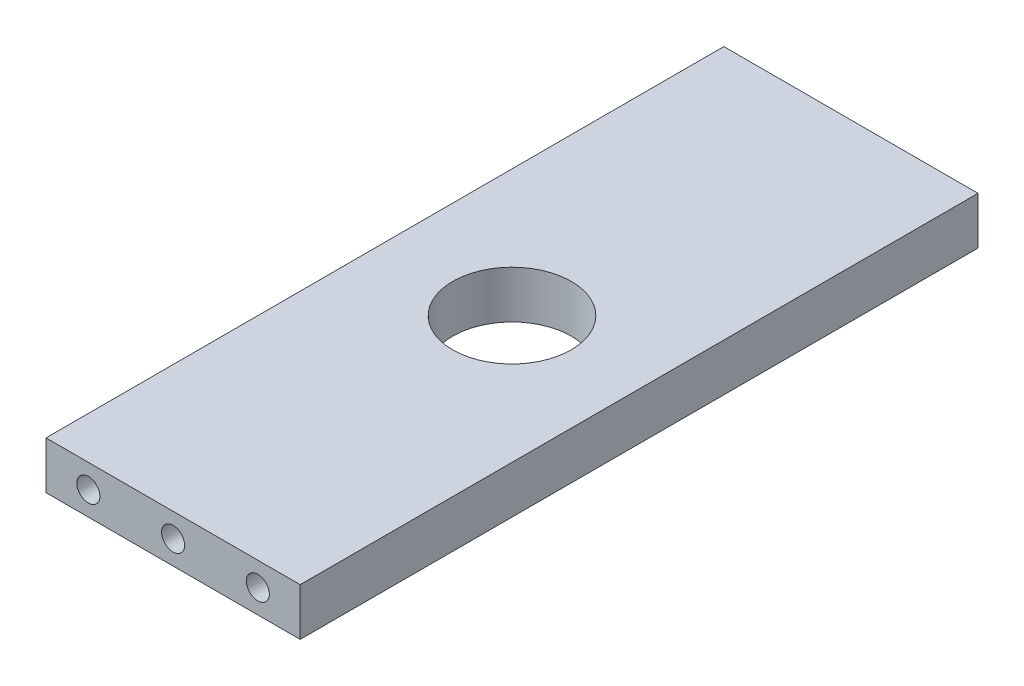
from build123d import *

# Parameters (mm, degrees)
SKETCH1_W             = 75
SKETCH1_H             = 14
BOSS_EXTRUDE1_DEPTH   = 200
SKETCH2_R             = 17.5
CUT_EXTRUDE1_DEPTH    = 226.39507559
M8_TAPPED_HOLE2_D     = 6.8
M8_TAPPED_HOLE2_DEPTH = 22.25
M8_TAPPED_HOLE2_TIP   = 2.042926105
M8_TAPPED_HOLE3_D     = 6.8
M8_TAPPED_HOLE3_DEPTH = 22.25
M8_TAPPED_HOLE3_TIP   = 2.042926105


with BuildPart() as part:
    # Sketch1 → Boss-Extrude1 (new body)
    with BuildSketch(Plane.XY):
        with Locations((65.49, 327)):
            Rectangle(SKETCH1_W, SKETCH1_H)
    extrude(amount=BOSS_EXTRUDE1_DEPTH)

    # Sketch2 → Cut-Extrude1 (cut, through all)
    with BuildSketch(Plane(origin=(0, 334, 0), x_dir=(1, 0, 0), z_dir=(0, 1, 0))):
        with Locations(Location((65.49, -100, 0), (0, 0, 270))):
            Circle(SKETCH2_R)
    extrude(amount=-CUT_EXTRUDE1_DEPTH, mode=Mode.SUBTRACT)

    # M8 Tapped Hole2
    with Locations(Plane.XY.offset(200)):
        with Locations((65.49, 327), (40.49, 327), (90.49, 327)):
            Hole(M8_TAPPED_HOLE2_D / 2, depth=M8_TAPPED_HOLE2_DEPTH)
            with Locations((0, 0, -(M8_TAPPED_HOLE2_DEPTH + M8_TAPPED_HOLE2_TIP / 2))):  # 118° drill point
                Cone(0, M8_TAPPED_HOLE2_D / 2, M8_TAPPED_HOLE2_TIP, mode=Mode.SUBTRACT)

    # M8 Tapped Hole3
    with Locations(Plane(origin=(0, 0, 0), x_dir=(-1, 0, 0), z_dir=(0, 0, -1))):
        with Locations((-90.49, 327), (-65.49, 327), (-40.49, 327)):
            Hole(M8_TAPPED_HOLE3_D / 2, depth=M8_TAPPED_HOLE3_DEPTH)
            with Locations((0, 0, -(M8_TAPPED_HOLE3_DEPTH + M8_TAPPED_HOLE3_TIP / 2))):  # 118° drill point
                Cone(0, M8_TAPPED_HOLE3_D / 2, M8_TAPPED_HOLE3_TIP, mode=Mode.SUBTRACT)


solid = part.part
